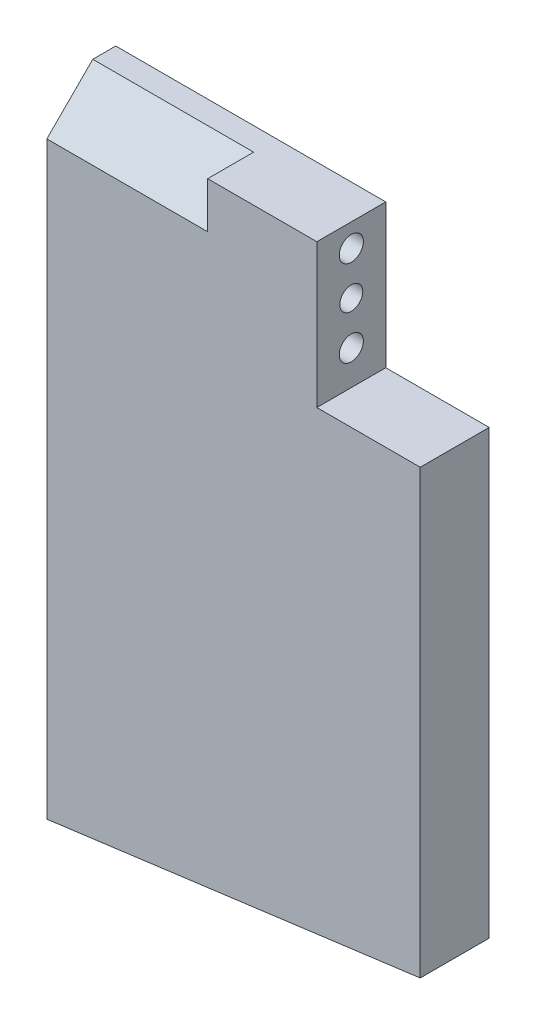
from build123d import *

# Parameters (mm, degrees)
SKETCH1_W                    = 65
SKETCH1_H                    = 12
BOSS_EXTRUDE1_DEPTH          = 51
BOSS_EXTRUDE2_DEPTH          = 12
SKETCH3_W                    = 18
SKETCH3_H                    = 25
CUT_EXTRUDE2_DEPTH           = 69.900909755
M5_TAPPED_HOLE1_D            = 4.2
M5_TAPPED_HOLE1_DEPTH        = 12.4
M5_TAPPED_HOLE1_TIP          = 1.2618073
M5_TAPPED_HOLE2_D            = 4.2
M5_TAPPED_HOLE2_DEPTH        = 12.4
M5_TAPPED_HOLE2_TIP          = 1.2618073
M5_TAPPED_HOLE3_D            = 4.2
M5_TAPPED_HOLE3_DEPTH        = 12.4
M5_TAPPED_HOLE3_TIP          = 1.2618073
CUT_EXTRUDE3_DEPTH           = 28
F_4_0_4_DIAMETER_HOLE1_D     = 4
F_4_0_4_DIAMETER_HOLE1_DEPTH = 8
F_4_0_4_DIAMETER_HOLE1_TIP   = 1.201721238


with BuildPart() as part:
    # Sketch1 → Boss-Extrude1 (new, symmetric)
    with BuildSketch(Plane(origin=(0, 0, 0), x_dir=(1, 0, 0), z_dir=(0, 1, 0))):
        Rectangle(SKETCH1_W, SKETCH1_H)
    extrude(amount=BOSS_EXTRUDE1_DEPTH, both=True)

    # Sketch4 → Boss-Extrude2 (add)
    with BuildSketch(Plane.XY.offset(6)):
        Polygon((-32.5, -51), (32.5, -51), (-32.5, -59.557412343), align=None)
    extrude(amount=-BOSS_EXTRUDE2_DEPTH)

    # Sketch3 → Cut-Extrude2 (cut, through all)
    with BuildSketch(Plane.XY.offset(6)):
        with Locations((23.5, 38.5)):
            Rectangle(SKETCH3_W, SKETCH3_H)
    extrude(amount=-CUT_EXTRUDE2_DEPTH, mode=Mode.SUBTRACT)

    # M5 Tapped Hole1
    with Locations(Plane(origin=(7.153590973, -54.336918053, 0), x_dir=(-0.9914448613738113, -0.13052619222004513, 0), z_dir=(0.13052619222004513, -0.9914448613738113, 0))):
        with Locations((-18.065122191, 0), (6.934877809, 0), (31.934877809, 0)):
            Hole(M5_TAPPED_HOLE1_D / 2, depth=M5_TAPPED_HOLE1_DEPTH)
            with Locations((0, 0, -(M5_TAPPED_HOLE1_DEPTH + M5_TAPPED_HOLE1_TIP / 2))):  # 118° drill point
                Cone(0, M5_TAPPED_HOLE1_D / 2, M5_TAPPED_HOLE1_TIP, mode=Mode.SUBTRACT)

    # M5 Tapped Hole2
    with Locations(Plane.ZY.offset(32.5)):
        with Locations((0, 43), (0, 3), (0, -37)):
            Hole(M5_TAPPED_HOLE2_D / 2, depth=M5_TAPPED_HOLE2_DEPTH)
            with Locations((0, 0, -(M5_TAPPED_HOLE2_DEPTH + M5_TAPPED_HOLE2_TIP / 2))):  # 118° drill point
                Cone(0, M5_TAPPED_HOLE2_D / 2, M5_TAPPED_HOLE2_TIP, mode=Mode.SUBTRACT)

    # M5 Tapped Hole3
    with Locations(Plane(origin=(14.5, 0, 0), x_dir=(0, 0, -1), z_dir=(1, 0, 0))):
        with Locations((0, 47), (0, 32)):
            Hole(M5_TAPPED_HOLE3_D / 2, depth=M5_TAPPED_HOLE3_DEPTH)
            with Locations((0, 0, -(M5_TAPPED_HOLE3_DEPTH + M5_TAPPED_HOLE3_TIP / 2))):  # 118° drill point
                Cone(0, M5_TAPPED_HOLE3_D / 2, M5_TAPPED_HOLE3_TIP, mode=Mode.SUBTRACT)

    # Sketch12 → Cut-Extrude3 (cut)
    with BuildSketch(Plane.ZY.offset(32.5)):
        Polygon((-2, 51), (6, 51), (6, 43), align=None)
    extrude(amount=-CUT_EXTRUDE3_DEPTH, mode=Mode.SUBTRACT)

    # Ø4.0 (4) Diameter Hole1
    with Locations(Plane(origin=(14.5, 0, 0), x_dir=(0, 0, -1), z_dir=(1, 0, 0))):
        with Locations((0, 39.5)):
            Hole(F_4_0_4_DIAMETER_HOLE1_D / 2, depth=F_4_0_4_DIAMETER_HOLE1_DEPTH)
            with Locations((0, 0, -(F_4_0_4_DIAMETER_HOLE1_DEPTH + F_4_0_4_DIAMETER_HOLE1_TIP / 2))):  # 118° drill point
                Cone(0, F_4_0_4_DIAMETER_HOLE1_D / 2, F_4_0_4_DIAMETER_HOLE1_TIP, mode=Mode.SUBTRACT)


solid = part.part
